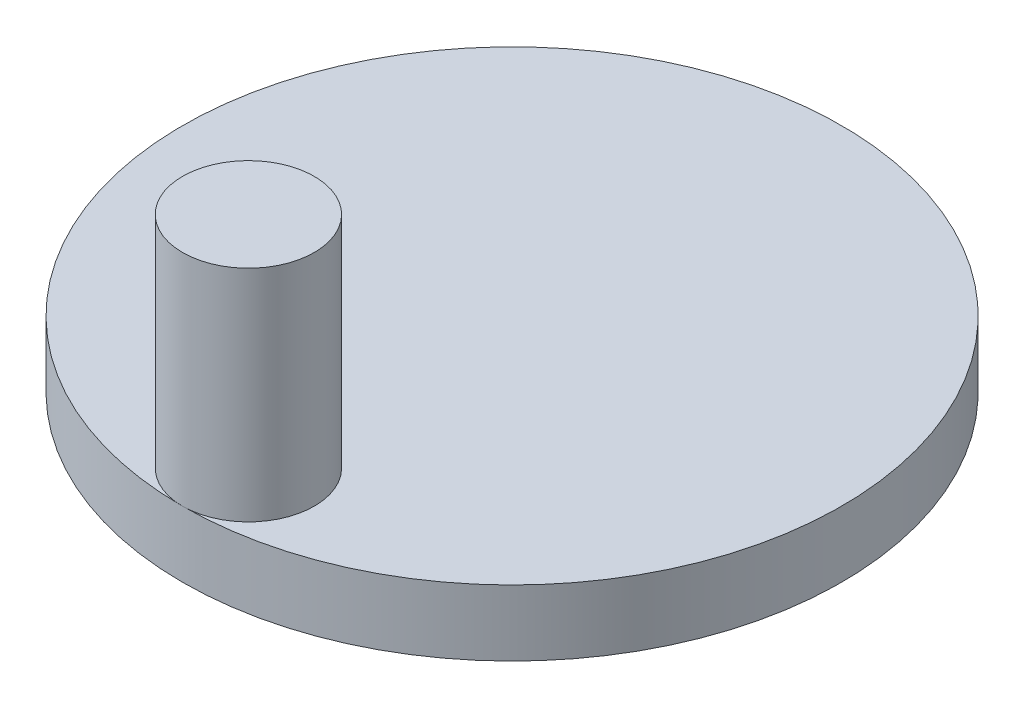
SolidWorks part; units mm, degrees
ref_plane "Front Plane" through (0, 0, 0) normal (0, 0, 1) x (1, 0, 0)
ref_plane "Top Plane" through (0, 0, 0) normal (0, 1, 0) x (1, 0, 0)
ref_plane "Right Plane" through (0, 0, 0) normal (1, 0, 0) x (0, 0, -1)
other "Configuration Table"
sketch "Sketch1" plane through (0, 0, 0) normal (0, 1, 0) x (1, 0, 0)
  circle A0 centre (0, 0) radius 15
  dimension "D1" = 30
extrude "Boss-Extrude1" add sketch "Sketch1" along normal blind 3
sketch "Sketch2" plane through (0, 3, 0) normal (0, 1, 0) x (1, 0, 0)
  circle A0 centre (0, -12) radius 3
  circle A1 centre (0, 0) radius 15 construction
  dimension "D1" = 6
extrude "Boss-Extrude2" add sketch "Sketch2" along normal blind 10
sketch "Sketch3" plane through (0, 0, 0) normal (0, -1, 0) x (-1, 0, 0)
  circle A0 centre (0, 0) radius 5
  dimension "D1" = 10
extrude "Boss-Extrude3" add sketch "Sketch3" along normal blind 2
sketch "Sketch4" plane through (0, -2, 0) normal (0, -1, 0) x (-1, 0, 0)
  line L1 (2, 2) -> (-2, 2)
  line L2 (2, 2) -> (2, -2)
  line L3 (2, -2) -> (-2, -2)
  line L4 (-2, 2) -> (-2, -2)
  line L5 (0, -2) -> (0, 2) construction
  line L6 (2, 0) -> (-2, 0) construction
  circle A1 centre (0, 0) radius 5
  circle A2 centre (0, 0) radius 5
  point P0 (0, 0)
  dimension "D1" = 4
  dimension "D2" = 0
extrude "Boss-Extrude4" add sketch "Sketch4" along normal blind 5
sketch "Sketch5" plane through (0, 0, 0) normal (0, -1, 0) x (-1, 0, 0)
  circle A0 centre (0, 0) radius 7.5
  dimension "D1" = 15
extrude "Boss-Extrude5" add sketch "Sketch5" along normal blind 2
